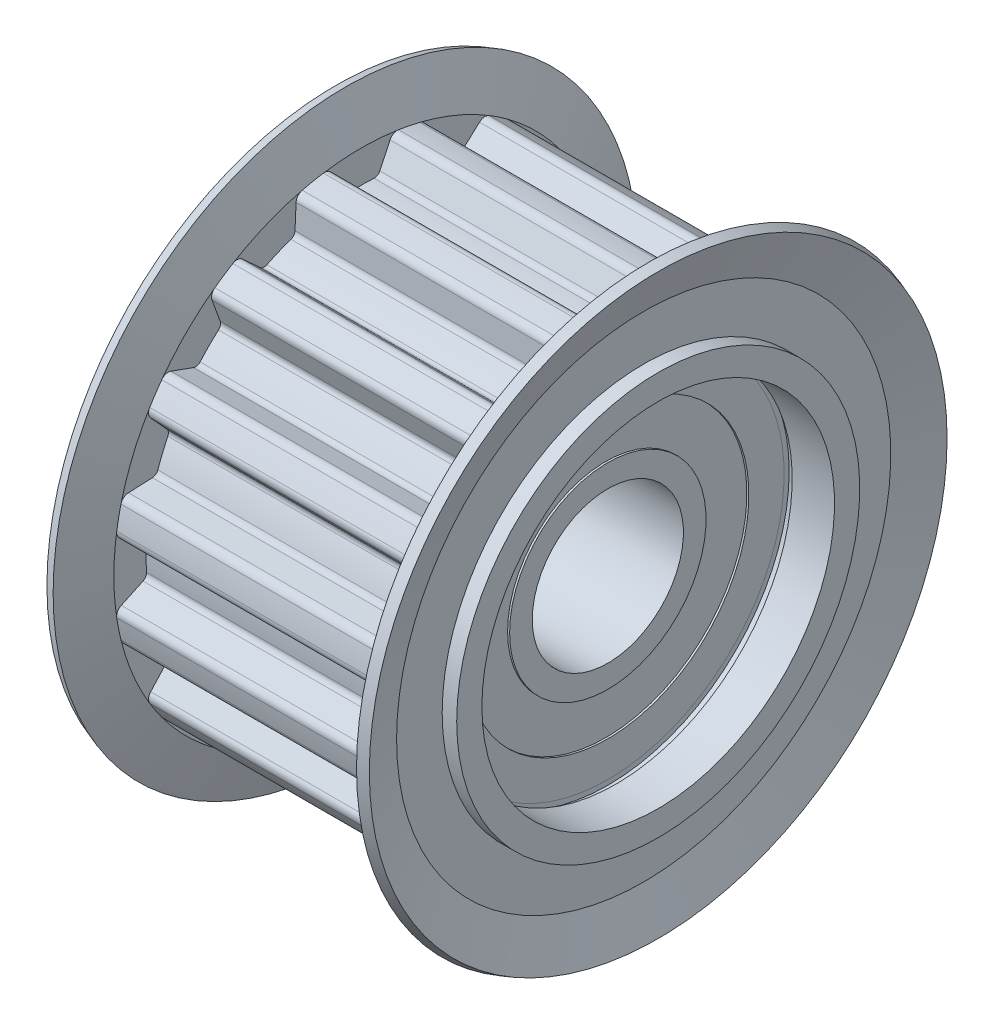
from build123d import *

# Parameters (mm, degrees)
CUT_EXTRUDE1_START = -32
CUT_EXTRUDE1_DEPTH = 32
CIRPATTERN1_COUNT  = 16


with BuildPart() as part:
    # Sketch1 → Revolve1 (revolve)
    with BuildSketch(Plane.XY, mode=Mode.PRIVATE) as revolve1_sk:
        Polygon((-16, 17), (-16, 20), (-13.5, 20), (-13.5, 24.525), (13.5, 24.525), (13.5, 20), (16, 20), (16, 17.5), (11.8, 17.5), (11.8, 18), (11, 18), (11, 17.5), (-11, 17.5), (-11, 17), align=None)
    revolve(revolve1_sk.sketch.rotate(Axis((-68.411960133, 0, 0), (1, 0, 0)), 90), axis=Axis((-68.411960133, 0, 0), (1, 0, 0)))

    # Sketch2 → Cut-Extrude1 (cut)
    with BuildSketch(Plane.ZY.offset(13.5).offset(CUT_EXTRUDE1_START)):
        with BuildLine():
            Line((-2.879978201, 23.787602575), (-1.874346267, 21.631017932))
            ThreePointArc((-1.874346267, 21.631017932), (-1.637430837, 21.369000616), (-1.294149419, 21.28569478))
            ThreePointArc((-1.294149419, 21.28569478), (0, 21.325), (1.294149419, 21.28569478))
            ThreePointArc((1.294149419, 21.28569478), (1.637430837, 21.369000616), (1.874346267, 21.631017932))
            Line((1.874346267, 21.631017932), (2.879978201, 23.787602575))
            ThreePointArc((2.879978201, 23.787602575), (3.227845319, 24.155011983), (3.726584791, 24.240218456))
            ThreePointArc((3.726584791, 24.240218456), (0, 24.525), (-3.726584791, 24.240218456))
            ThreePointArc((-3.726584791, 24.240218456), (-3.227845319, 24.155011983), (-2.879978201, 23.787602575))
        make_face()
    cut_extrude1 = extrude(amount=CUT_EXTRUDE1_DEPTH, mode=Mode.SUBTRACT)

    # CirPattern1: Cut-Extrude1 ×16 about axis
    cirpattern1_axis = Axis((0, 0, 0), (1, 0, 0))
    for i in range(1, CIRPATTERN1_COUNT):
        add(cut_extrude1.rotate(cirpattern1_axis, i * 360 / CIRPATTERN1_COUNT), mode=Mode.SUBTRACT)

    # Sketch3 → Revolve2 (revolve)
    with BuildSketch(Plane.XY, mode=Mode.PRIVATE) as revolve2_sk:
        Polygon((-13.5, 20), (-13.5, 24.525), (-15.055431844, 29), (-16, 28.671684606), (-14.558684853, 24.525), (-14.558684853, 20), align=None)
    revolve(revolve2_sk.sketch.rotate(Axis((-8.744487855, 0, 0), (1, 0, 0)), 90), axis=Axis((-8.744487855, 0, 0), (1, 0, 0)))

    # Sketch4 → Revolve3 (revolve)
    with BuildSketch(Plane.XY, mode=Mode.PRIVATE) as revolve3_sk:
        Polygon((13.5, 20), (13.5, 24.525), (15.055431844, 29), (16, 28.671684606), (14.558684853, 24.525), (14.558684853, 20), align=None)
    revolve(revolve3_sk.sketch.rotate(Axis((-8.744487855, 0, 0), (1, 0, 0)), 90), axis=Axis((-8.744487855, 0, 0), (1, 0, 0)))


with BuildPart() as body_2:
    # Sketch5 → Revolve5 (revolve)
    with BuildSketch(Plane.XY, mode=Mode.PRIVATE) as revolve5_sk:
        Polygon((-11, 7.5), (-11, 9.75), (-10.8, 9.75), (-10.8, 14), (-11, 14), (-11, 17.5), (11, 17.5), (11, 14), (10.8, 14), (10.8, 9.75), (11, 9.75), (11, 7.5), align=None)
    revolve(revolve5_sk.sketch.rotate(Axis((-8.744487855, 0, 0), (1, 0, 0)), 90), axis=Axis((-8.744487855, 0, 0), (1, 0, 0)))


solid = Compound([part.part, body_2.part])
